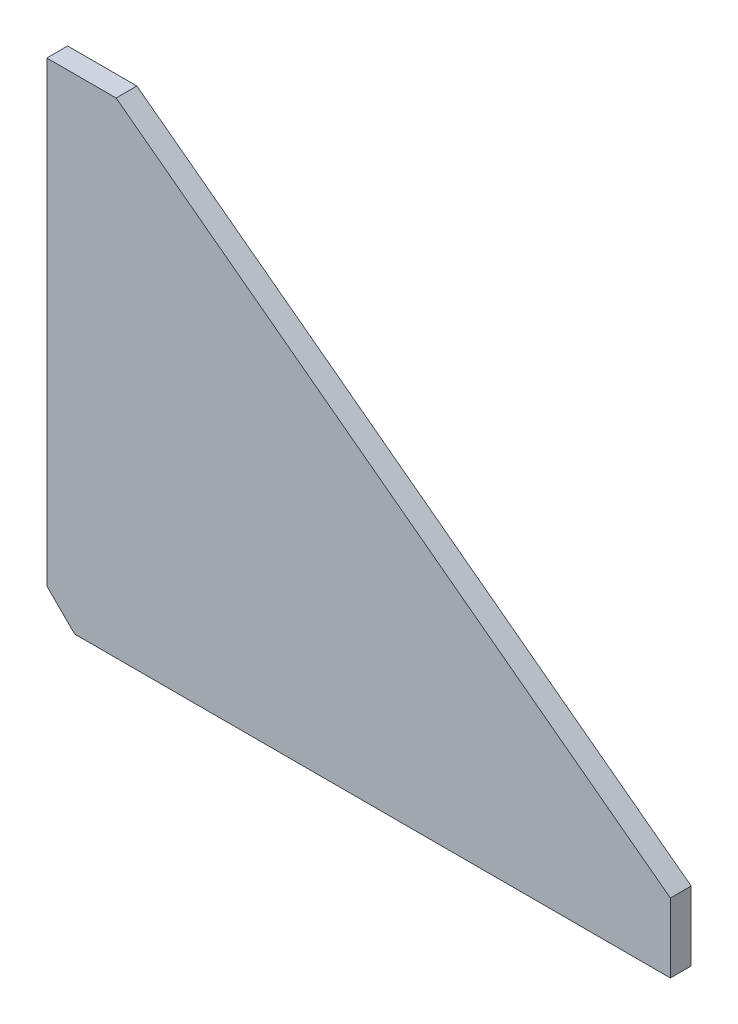
SolidWorks part; units mm, degrees
material "1023 Carbon Steel Plate (SS)"
ref_plane "Front Plane" through (0, 0, 0) normal (0, 0, 1) x (1, 0, 0)
ref_plane "Top Plane" through (0, 0, 0) normal (0, 1, 0) x (1, 0, 0)
ref_plane "Right Plane" through (0, 0, 0) normal (1, 0, 0) x (0, 0, -1)
sketch "Sketch1" plane through (0, 0, 0) normal (0, 0, 1) x (1, 0, 0)
  line L3 (-17.5, 17.5) -> (22.5, -12.5)
  line L4 (-17.5, 17.5) -> (-22.5, 17.5)
  line L5 (22.5, -12.5) -> (22.5, -17.5)
  line L6 (22.5, -17.5) -> (-20.5, -17.5)
  line L7 (-22.5, 17.5) -> (-22.5, -15.5)
  line L8 (22.5, 17.5) -> (-22.5, -17.5) construction
  line L9 (22.5, -17.5) -> (-22.5, 17.5) construction
  line L10 (-20.5, -17.5) -> (-22.5, -15.5)
  point P0 (0, 0)
  dimension "D1" = 45
  dimension "D2" = 35
  dimension "D3" = 5
  dimension "D4" = 5
extrude "Boss-Extrude1" add sketch "Sketch1" along normal blind 1.5
